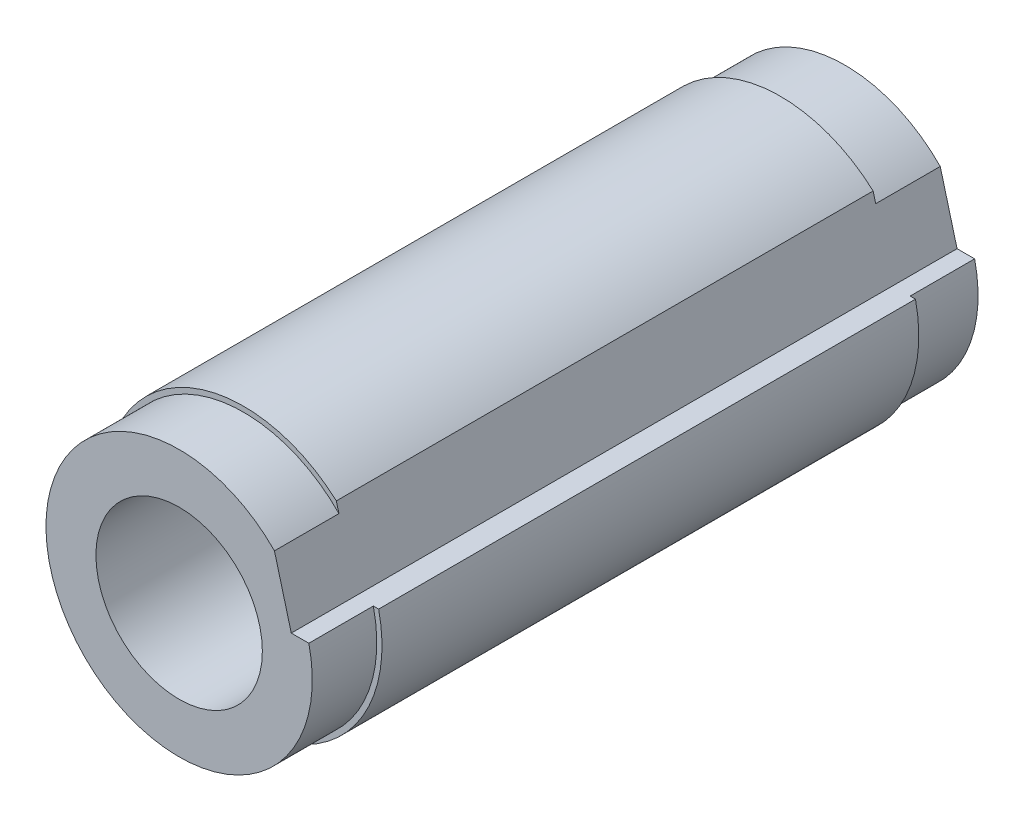
SolidWorks part; units mm, degrees
ref_plane "Front Plane" through (0, 0, 0) normal (0, 0, 1) x (1, 0, 0)
ref_plane "Top Plane" through (0, 0, 0) normal (0, 1, 0) x (1, 0, 0)
ref_plane "Right Plane" through (0, 0, 0) normal (1, 0, 0) x (0, 0, -1)
sketch "Sketch1" plane through (0, 0, 0) normal (0, 0, 1) x (1, 0, 0)
  circle A0 centre (0, 0) radius 36.5
  circle A1 centre (0, 0) radius 66.5
  dimension "D1" = 133
  dimension "D2" = 73
extrude "Boss-Extrude1" add sketch "Sketch1" along normal blind 320
sketch "Sketch3" plane through (0, 0, 320) normal (0, 0, 1) x (1, 0, 0)
  circle A0 centre (0, 0) radius 40
  dimension "D1" = 80
extrude "Cut-Extrude1" cut sketch "Sketch3" against normal blind 79.7
sketch "Sketch4" plane through (0, 0, 320) normal (0, 0, 1) x (1, 0, 0)
  circle A0 centre (0, 0) radius 64
  circle A1 centre (0, 0) radius 66.5 construction
  circle A2 centre (0, 0) radius 66.5
  dimension "D1" = 128
extrude "Cut-Extrude2" cut sketch "Sketch4" against normal blind 31
ref_plane "Plane1" through (0, 0, 160) normal (0, 0, 1) x (1, 0, 0)
mirror "Mirror1" about plane through (0, 0, 160) normal (0, 0, 1) of "Cut-Extrude1", "Cut-Extrude2"
sketch "Sketch5" plane through (0, 0, 320) normal (0, 0, 1) x (1, 0, 0)
  line L0 (0, 0) -> (109.6058, 0) construction
  line L1 (-16.2653, 14.5) -> (90.9666, 14.5) construction
  line L2 (64.8999, 14.5) -> (53.8999, 14.5)
  line L3 (53.8999, 14.5) -> (44.5581, 49.3642)
  circle A0 centre (0, 0) radius 66.5 construction
  arc A1 (64.8999, 14.5) -> (44.5581, 49.3642) centre (0, 0) ccw
  dimension "D2" = 11
  dimension "D1" = 14.5
  dimension "D3" = 105
extrude "Cut-Extrude3" cut sketch "Sketch5" against normal through all
